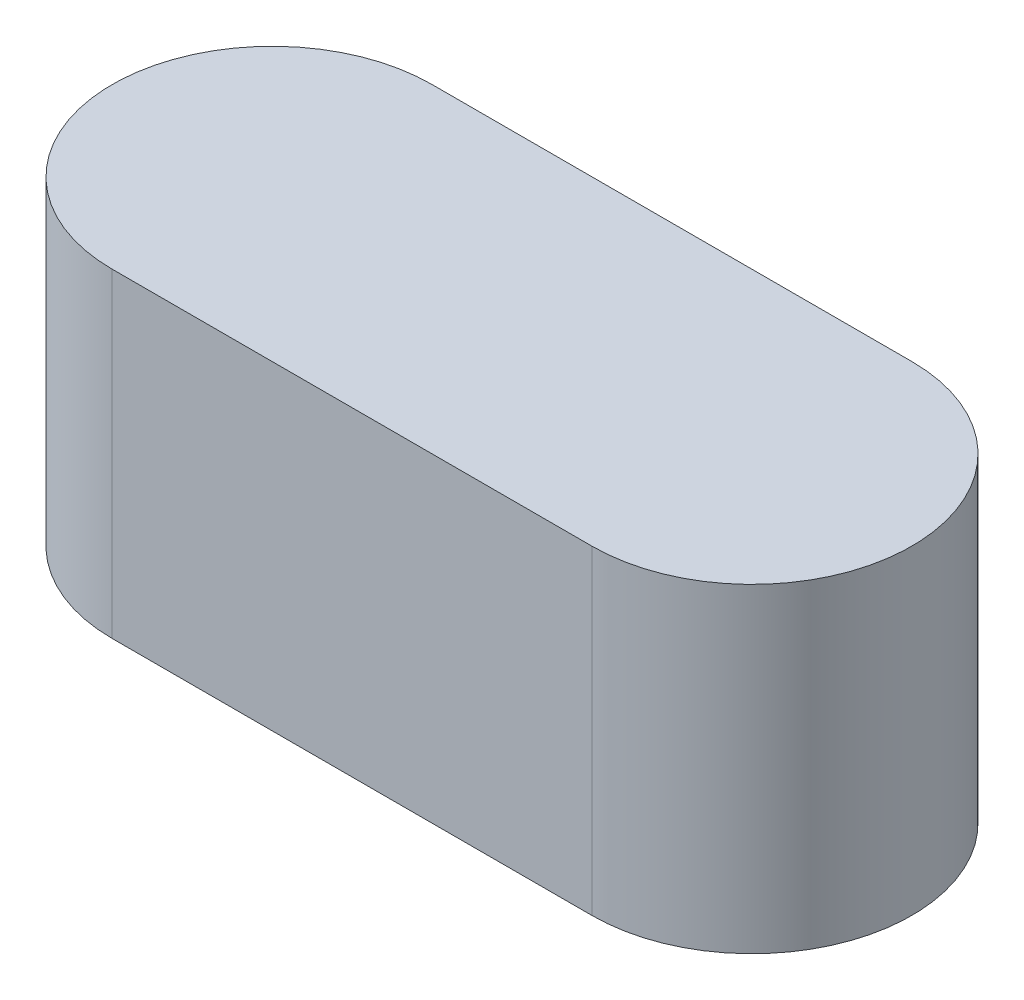
SolidWorks part; units mm, degrees
ref_plane "Front Plane" through (0, 0, 0) normal (0, 0, 1) x (1, 0, 0)
ref_plane "Top Plane" through (0, 0, 0) normal (0, 1, 0) x (1, 0, 0)
ref_plane "Right Plane" through (0, 0, 0) normal (1, 0, 0) x (0, 0, -1)
sketch "Sketch1" plane through (0, 0, 0) normal (0, 1, 0) x (1, 0, 0)
  line L0 (-75, 0) -> (75, 0) construction
  line L1 (-75, 50) -> (75, 50)
  line L2 (-75, -50) -> (75, -50)
  arc A0 (-75, 50) -> (-75, -50) centre (-75, 0) ccw
  arc A1 (75, -50) -> (75, 50) centre (75, 0) ccw
  point P3 (0, 0)
  dimension "D1" = 50
  dimension "D2" = 150
extrude "Boss-Extrude1" add sketch "Sketch1" along normal blind 100
